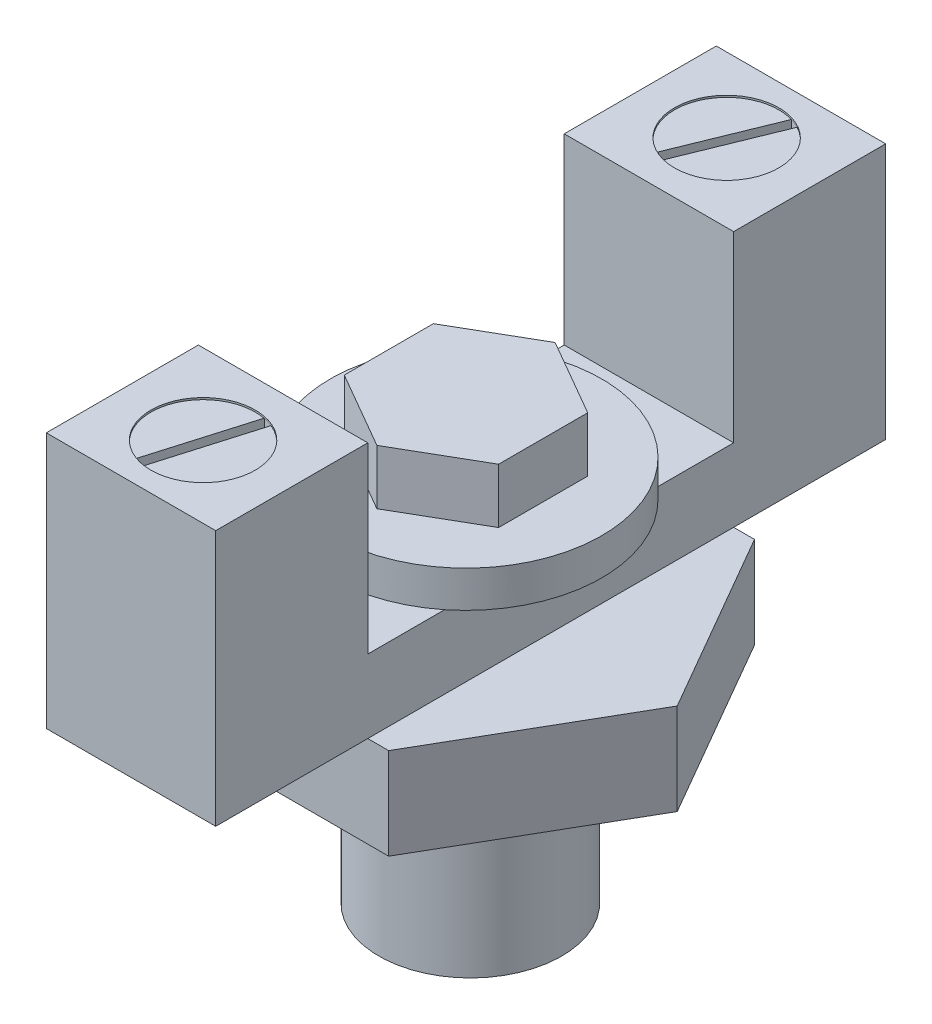
SolidWorks part; units mm, degrees
ref_plane "Front Plane" through (0, 0, 0) normal (0, 0, 1) x (1, 0, 0)
ref_plane "Top Plane" through (0, 0, 0) normal (0, 1, 0) x (1, 0, 0)
ref_plane "Right Plane" through (0, 0, 0) normal (1, 0, 0) x (0, 0, -1)
sketch "Sketch1" plane through (0, 0, 0) normal (0, 1, 0) x (1, 0, 0)
  line L1 (5.7735, 10) -> (-5.7735, 10)
  line L2 (-5.7735, 10) -> (-11.547, 0)
  line L3 (-11.547, 0) -> (-5.7735, -10)
  line L4 (-5.7735, -10) -> (5.7735, -10)
  line L5 (5.7735, -10) -> (11.547, 0)
  line L6 (11.547, 0) -> (5.7735, 10)
  circle A0 centre (0, 0) radius 10 construction
  dimension "D1" = 20
extrude "Boss-Extrude1" add sketch "Sketch1" along normal blind 5
sketch "Sketch2" plane through (0, 0, 0) normal (0, -1, 0) x (1, 0, 0)
  circle A0 centre (0.2348, 0) radius 5
  dimension "D1" = 10
extrude "Boss-Extrude2" add sketch "Sketch2" along normal blind 10
sketch "Sketch3" plane through (0, 5, 0) normal (0, 1, 0) x (1, 0, 0)
  line L1 (-4.6309, -18.3139) -> (4.6309, -18.3139)
  line L2 (-4.6309, -18.3139) -> (-4.6309, 18.3139)
  line L3 (-4.6309, 18.3139) -> (4.6309, 18.3139)
  line L4 (4.6309, -18.3139) -> (4.6309, 18.3139)
  line L5 (-4.6309, -18.3139) -> (4.6309, 18.3139) construction
  line L6 (-4.6309, 18.3139) -> (4.6309, -18.3139) construction
  point P0 (0, 0)
extrude "Boss-Extrude3" add sketch "Sketch3" along normal blind 4
sketch "Sketch4" plane through (0, 9, 0) normal (0, 1, 0) x (1, 0, 0)
  line L1 (-4.6309, 18.3139) -> (4.6309, 18.3139)
  line L2 (-4.6309, 18.3139) -> (-4.6309, 10)
  line L3 (-4.6309, 10) -> (4.6309, 10)
  line L4 (4.6309, 18.3139) -> (4.6309, 10)
  line L5 (-4.6309, -18.3139) -> (4.6309, -18.3139)
  line L6 (-4.6309, -18.3139) -> (-4.6309, -10)
  line L7 (-4.6309, -10) -> (4.6309, -10)
  line L8 (4.6309, -18.3139) -> (4.6309, -10)
extrude "Boss-Extrude4" add sketch "Sketch4" along normal blind 10
sketch "Sketch5" plane through (0, 9, 0) normal (0, 1, 0) x (1, 0, 0)
  circle A0 centre (0, 0) radius 7.424
extrude "Boss-Extrude5" add sketch "Sketch5" along normal blind 2
sketch "Sketch6" plane through (0, 11, 0) normal (0, 1, 0) x (1, 0, 0)
  line L1 (0, 4.8711) -> (-4.2185, 2.4355)
  line L2 (-4.2185, 2.4355) -> (-4.2185, -2.4355)
  line L3 (-4.2185, -2.4355) -> (0, -4.8711)
  line L4 (0, -4.8711) -> (4.2185, -2.4355)
  line L5 (4.2185, -2.4355) -> (4.2185, 2.4355)
  line L6 (4.2185, 2.4355) -> (0, 4.8711)
  circle A0 centre (0, 0) radius 4.2185 construction
extrude "Boss-Extrude6" add sketch "Sketch6" along normal blind 3
sketch "Sketch7" plane through (0, 19, 0) normal (0, 1, 0) x (1, 0, 0)
  circle A0 centre (0, 14.2505) radius 2.8507
  circle A1 centre (0, -14.3728) radius 2.8507
extrude "Cut-Extrude1" cut sketch "Sketch7" against normal blind 0.1
sketch "Sketch8" plane through (0, 18.9, 0) normal (0, 1, 0) x (1, 0, 0)
  line L0 (-1.3431, 11.7193) -> (0.8043, 17.0008)
  line L1 (-1.3431, 11.7193) -> (-0.8167, 11.5053)
  line L2 (0.8043, 17.0008) -> (1.3307, 16.7868)
  line L3 (-0.8167, 11.5053) -> (1.3307, 16.7868)
  line L4 (-1.3431, 11.7193) -> (1.3307, 16.7868) construction
  line L5 (0.8043, 17.0008) -> (-0.8167, 11.5053) construction
  line L6 (-1.0769, -17.0275) -> (0.5318, -11.5578)
  line L7 (-1.0769, -17.0275) -> (-0.5318, -17.1878)
  line L8 (0.5318, -11.5578) -> (1.0769, -11.7181)
  line L9 (-0.5318, -17.1878) -> (1.0769, -11.7181)
  line L10 (-1.0769, -17.0275) -> (1.0769, -11.7181) construction
  line L11 (0.5318, -11.5578) -> (-0.5318, -17.1878) construction
  point P1 (-0.0062, 14.253)
  point P2 (0, -14.3728)
extrude "Cut-Extrude2" cut sketch "Sketch8" against normal blind 1
